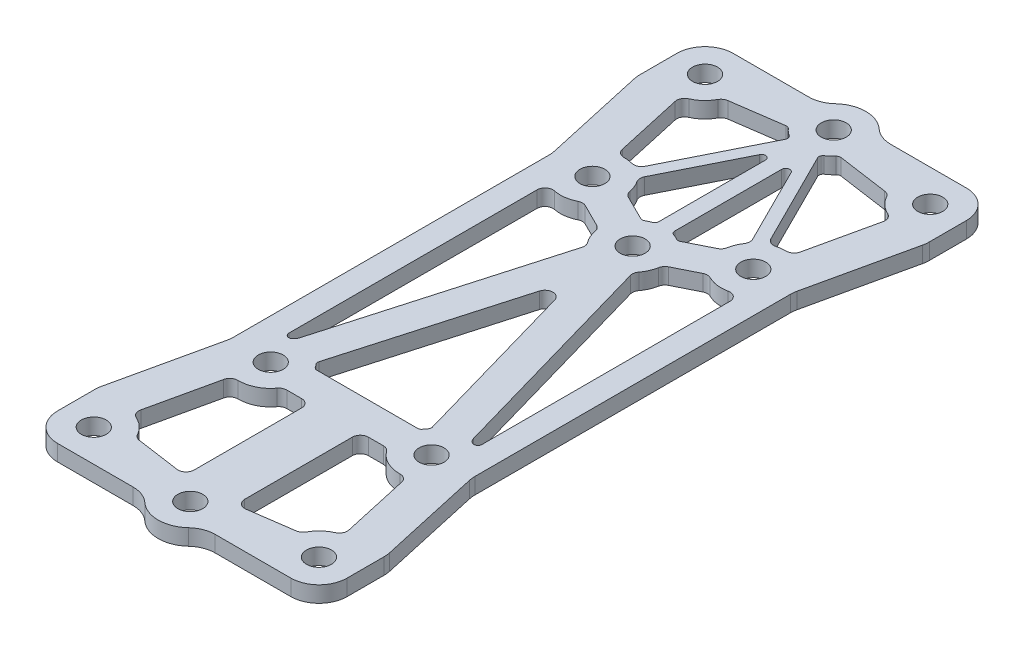
SolidWorks part; units mm, degrees
material "Thornel Mat VMA"
ref_plane "前视基准面" through (0, 0, 0) normal (0, 0, 1) x (1, 0, 0)
ref_plane "上视基准面" through (0, 0, 0) normal (0, 1, 0) x (1, 0, 0)
ref_plane "右视基准面" through (0, 0, 0) normal (1, 0, 0) x (0, 0, -1)
other "Configuration Table"
sketch "草图3" plane through (0, 0, 0) normal (0, 1, 0) x (1, 0, 0)
  line L0 (10, -34.1992) -> (10, 52.6309) construction
  line L1 (0, 0) -> (31.1432, 0) construction
  line L6 (-14, 38) -> (14, 38) construction
  line L7 (-14, 38) -> (-14, -38) construction
  line L8 (-14, -38) -> (14, -38) construction
  line L9 (14, 38) -> (14, -38) construction
  line L10 (-14, 38) -> (14, -38) construction
  line L11 (-14, -38) -> (14, 38) construction
  line L12 (-18, -42) -> (18, -42)
  line L13 (-18, -42) -> (-18, 42)
  line L14 (-18, 42) -> (18, 42)
  line L15 (18, -42) -> (18, 42)
  line L16 (-18, -42) -> (18, 42) construction
  line L17 (-18, 42) -> (18, -42) construction
  line L18 (6, 62.0596) -> (6, -48.8242) construction
  line L19 (0, 0) -> (0, -11.1844) construction
  circle A7 centre (14, 38) radius 1.55
  circle A8 centre (-14, 38) radius 1.55
  circle A9 centre (-14, -38) radius 1.55
  circle A10 centre (14, -38) radius 1.55
  circle A11 centre (0, 15) radius 1.55
  circle A12 centre (10, -20) radius 1.55
  circle A15 centre (0, 40) radius 1.55
  circle A17 centre (0, 40) radius 4
  circle A19 centre (0, -40) radius 1.55
  circle A20 centre (0, -40) radius 4
  circle A26 centre (-10, -20) radius 1.55
  circle A27 centre (-10, 20) radius 1.55
  circle A28 centre (10, 20) radius 1.55
  point P14 (0, 0)
  point P42 (0, 0)
  dimension "D2" = 6
  dimension "D4" = 20
  dimension "D5" = 15
  dimension "D9" = 3.1
  dimension "D12" = 4
  dimension "D13" = 8
  dimension "D14" = 2
  dimension "D3" = 3.1
  dimension "D6" = 10
  dimension "D7" = 4
  dimension "D8" = 76
  dimension "D10" = 28
  dimension "D11" = 4
extrude "凸台-拉伸1" add sketch "草图3" along normal blind 2
sketch "草图4" plane through (0, 2, 0) normal (0, 1, 0) x (1, 0, 0)
  line L5 (-14, 38) -> (0, 40)
  line L6 (0, 40) -> (14, 38)
  line L7 (14, 38) -> (10, 20)
  line L8 (10, 20) -> (0, 15)
  line L14 (0, 15) -> (-10, 20)
  line L15 (-10, 20) -> (-14, 38)
  line L16 (-10, 20) -> (0, 40)
  line L17 (10, 20) -> (0, 40)
  line L18 (0, 15) -> (0, 40)
  line L22 (-10, -20) -> (10, -20)
  line L23 (10, -20) -> (14, -38)
  line L24 (14, -38) -> (0, -40)
  line L26 (0, -40) -> (-14, -38)
  line L27 (-10.2879, -36.51) -> (-3.1464, -37.5302)
  line L28 (-14, -38) -> (-10, -20)
  line L29 (0, 15) -> (-10, -20)
  line L30 (-10, 20) -> (-10, -20)
  line L31 (0, 15) -> (10, -20)
  line L32 (10, -20) -> (10, 20)
  line L33 (-0.3167, 36.0126) -> (-7, 22.6458)
  line L34 (-1, 34.6459) -> (-1, 18.873)
  line L35 (-6.0072, 20.2397) -> (-2.204, 18.338)
  line L36 (6.0072, 20.2397) -> (2.204, 18.338)
  line L37 (1, 34.6459) -> (1, 18.873)
  line L38 (0.3167, 36.0126) -> (7, 22.6458)
  line L39 (-15.2009, 34.1845) -> (-12.7038, 22.9478)
  line L40 (-7.796, 16.662) -> (-3.9928, 14.7603)
  line L41 (7.796, 16.662) -> (3.9928, 14.7603)
  line L42 (15.2009, 34.1845) -> (12.7038, 22.9478)
  line L43 (-10.2879, 36.51) -> (-3.1464, 37.5302)
  line L44 (10.2879, 36.51) -> (3.1464, 37.5302)
  line L45 (-12, 16.5359) -> (-12, -16.5359)
  line L46 (-10.9714, -16.1197) -> (-2.8747, 12.2186)
  line L47 (-7.1253, -17.2186) -> (0.9714, 11.1197)
  line L48 (7.1253, -17.2186) -> (-0.9714, 11.1197)
  line L49 (10.9714, -16.1197) -> (2.8747, 12.2186)
  line L50 (12, 16.5359) -> (12, -16.5359)
  line L51 (-15.2009, -34.1845) -> (-12.7038, -22.9478)
  line L52 (-6.5359, -18) -> (6.5359, -18)
  line L53 (-6.5359, -22) -> (6.5359, -22)
  line L54 (0, -40) -> (0, -20)
  line L55 (-3.1464, -20) -> (-3.1464, -37.5302)
  line L56 (10.2879, -36.51) -> (3.1464, -37.5302)
  line L57 (3.1464, -20) -> (3.1464, -37.5302)
  line L58 (15.2009, -34.1845) -> (12.7038, -22.9478)
  line L59 (18, 33.5) -> (15, 20)
  line L60 (18, -42) -> (18, 42) construction
  line L61 (15, 20) -> (15, -20)
  line L62 (15, -20) -> (18, -33.5)
  line L63 (-15, -20) -> (-18, -33.5)
  line L64 (-15, 20) -> (-15, -20)
  line L65 (-18, 33.5) -> (-15, 20)
  circle A29 centre (14, -38) radius 1.55 construction
  circle A30 centre (0, -40) radius 1.55 construction
  circle A31 centre (-14, -38) radius 1.55 construction
  circle A32 centre (10, -20) radius 1.55 construction
  circle A33 centre (-10, -20) radius 1.55 construction
  circle A34 centre (-10, 20) radius 1.55 construction
  circle A35 centre (0, 15) radius 1.55 construction
  circle A36 centre (10, 20) radius 1.55 construction
  circle A37 centre (14, 38) radius 1.55 construction
  circle A38 centre (0, 40) radius 1.55 construction
  circle A39 centre (-14, 38) radius 1.55 construction
  circle A40 centre (14, -38) radius 1.55
  circle A41 centre (0, -40) radius 1.55
  circle A42 centre (-14, -38) radius 1.55
  circle A43 centre (10, -20) radius 1.55
  circle A44 centre (-10, -20) radius 1.55
  circle A45 centre (-10, 20) radius 1.55
  circle A46 centre (0, 15) radius 1.55
  circle A47 centre (10, 20) radius 1.55
  circle A48 centre (14, 38) radius 1.55
  circle A49 centre (0, 40) radius 1.55
  circle A50 centre (-14, 38) radius 1.55
  circle A51 centre (0, 40) radius 4
  circle A52 centre (14, 38) radius 4
  circle A53 centre (-14, 38) radius 4
  circle A54 centre (-10, 20) radius 4
  circle A55 centre (0, 15) radius 4
  circle A56 centre (10, 20) radius 4
  circle A57 centre (10, -20) radius 4
  circle A58 centre (-10, -20) radius 4
  circle A59 centre (-14, -38) radius 4
  circle A60 centre (0, -40) radius 4
  circle A61 centre (14, -38) radius 4
  line M16 (18, -42) -> (18, 42)
  line M20 (-18, 42) -> (-18, -42)
  dimension "D1" = 8
  dimension "D6" = 2
  dimension "D14" = 4.5
  dimension "D2" = 1.5
  dimension "D3" = 1
  dimension "D4" = 2
  dimension "D5" = 2
  dimension "D7" = 2
  dimension "D8" = 2
  dimension "D9" = 2
  dimension "D10" = 2
  dimension "D12" = 2
  dimension "D13" = 3
  dimension "D15" = 4.5
extrude "切除-拉伸1" cut sketch "草图4" against normal through all and the other way through all contours A54 L16 A51 L43 A53 L15 | A55 L34 L33 A54 L35 | A56 L7 A52 L44 A51 L17 | A56 L38 L37 A55 L36 | A55 L40 A54 L30 L46 | A58 L52 A57 L48 L47 | A56 L41 A55 L49 L32 | A60 L55 L53 A58 L28 A59 L27 | A61 L23 A57 L53 L57 A60 L56 | A58 L46 L30 A54 L45 | A57 L50 A56 L32 L49 | L65 L63 L64 M20 | L61 L62 L59 M16
fillet "圆角1" radius 3.5 16 edges at (-18, 1, 42) (3.4641, 1, 42) (-3.4641, 1, 42) (18, 1, 42) (18, 1, -42) (-3.4641, 1, -42) (3.4641, 1, -42) (-18, 1, -42) (18, 1, -33.5) (15, 1, -20) (-18, 1, 33.5) (18, 1, 33.5) (15, 1, 20) (-15, 1, 20) (-15, 1, -20) (-18, 1, -33.5)
fillet "圆角4" radius 1 35 edges at (13.1323, 1, 34.0953) (10.8677, 1, 23.9047) (6.5359, 1, 22) (10.2879, 1, 36.51) (-10.2879, 1, 36.51) (-13.1323, 1, 34.0953) (-6.5359, 1, 22) (-10.8677, 1, 23.9047) (3.1464, 1, 22) (-3.1464, 1, 22) (10.9714, 1, 16.1197) (13.1323, 1, -34.0953) (10.2879, 1, -36.51) (10.8677, 1, -23.9047) (8.2111, 1, -23.5777) (7, 1, -22.6458) (6.0072, 1, -20.2397) (12, 1, -16.5359) (7.796, 1, -16.662) (2.8747, 1, -12.2186) (3.9928, 1, -14.7603) (0, 1, -7.7199) (-10.9714, 1, 16.1197) (-3.9928, 1, -14.7603) (-2.8747, 1, -12.2186) (-7.796, 1, -16.662) (-12, 1, -16.5359) (-6.0072, 1, -20.2397) (-7, 1, -22.6458) (-8.2111, 1, -23.5777) (-10.8677, 1, -23.9047) (-10.2879, 1, -36.51) (-13.1323, 1, -34.0953) (3.1464, 1, 37.5302) (-3.1464, 1, 37.5302)
fillet "圆角5" radius 0.5 16 edges at (-7.1253, 1, 17.2186) (-6.5359, 1, 18) (6.5359, 1, 18) (7.1253, 1, 17.2186) (12, 1, 16.5359) (-12, 1, 16.5359) (2.204, 1, -18.338) (1, 1, -18.873) (-1, 1, -18.873) (-2.204, 1, -18.338) (1, 1, -34.6459) (-1, 1, -34.6459) (3.1464, 1, -37.5302) (1.7889, 1, -36.4223) (-1.7889, 1, -36.4223) (-3.1464, 1, -37.5302)
